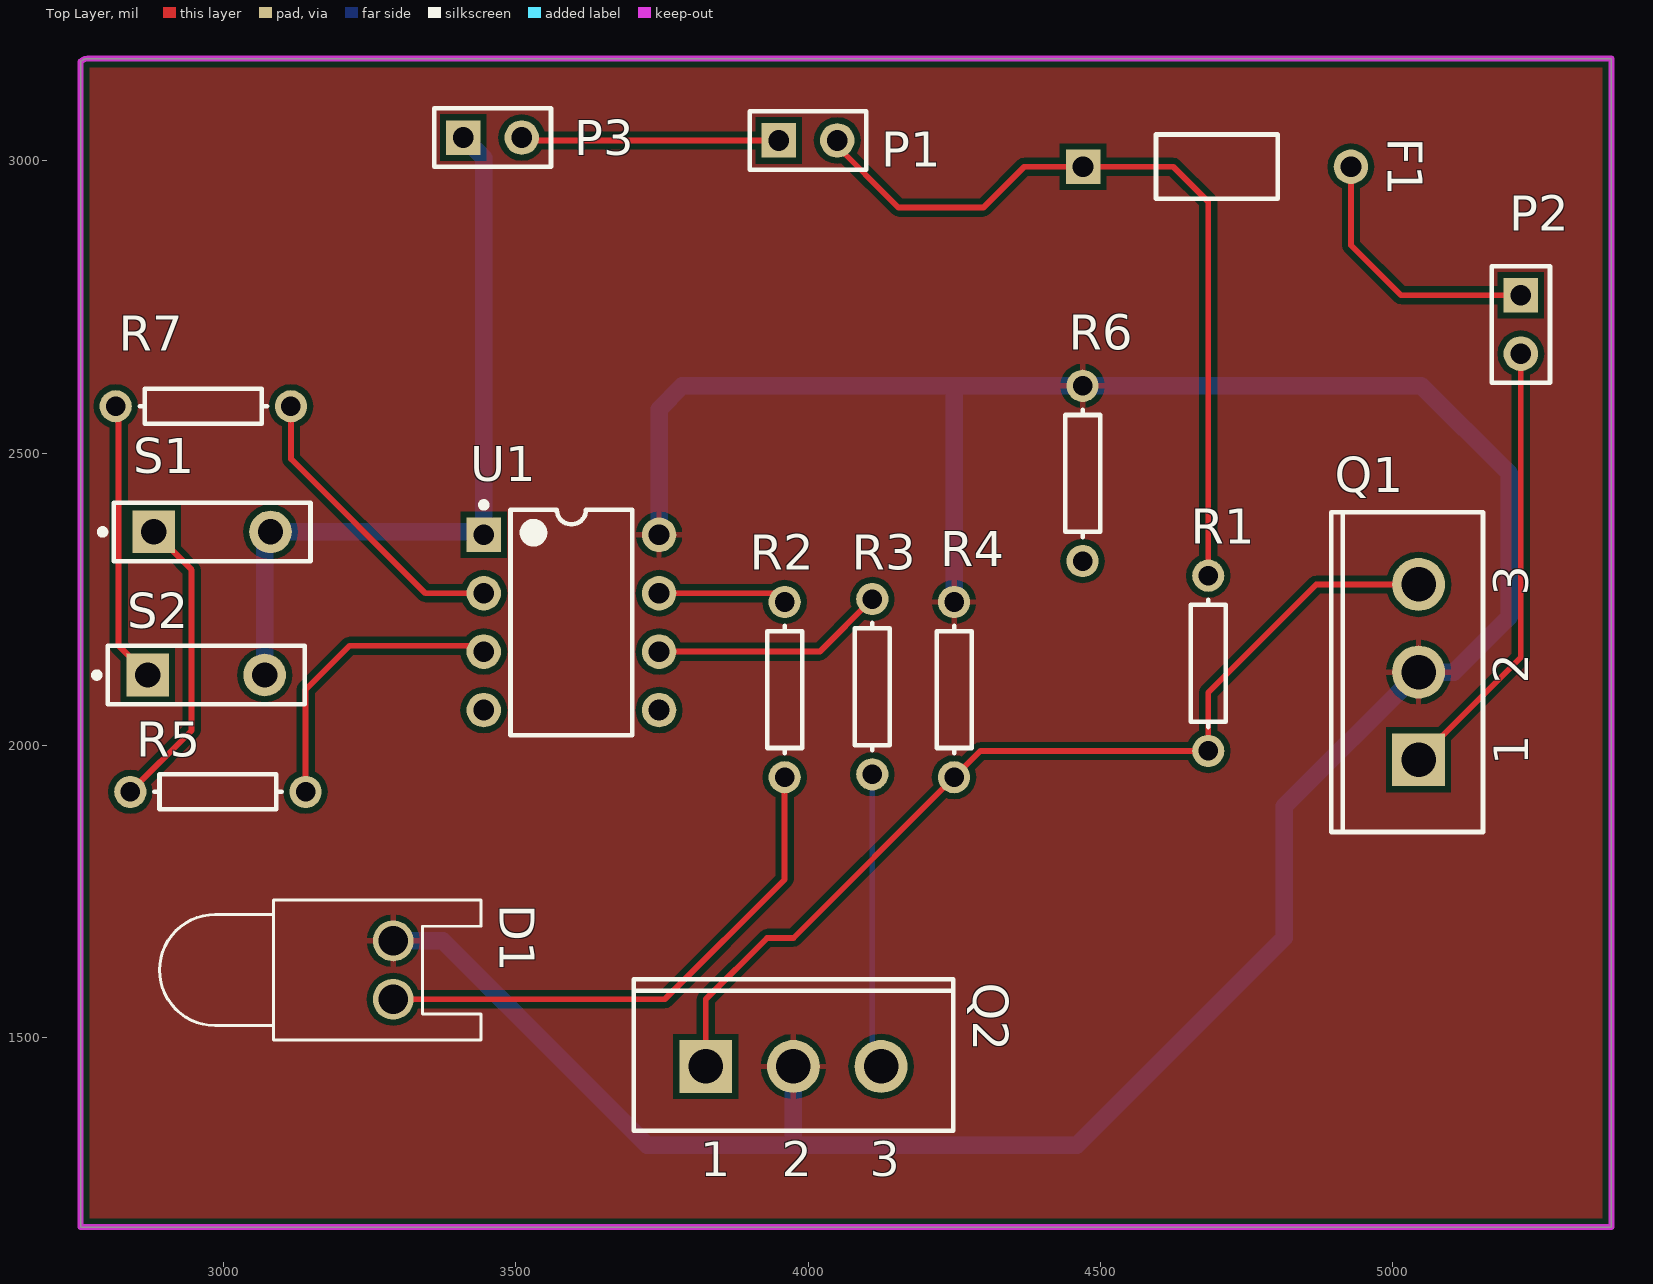
[diagram p0: Top Layer view]
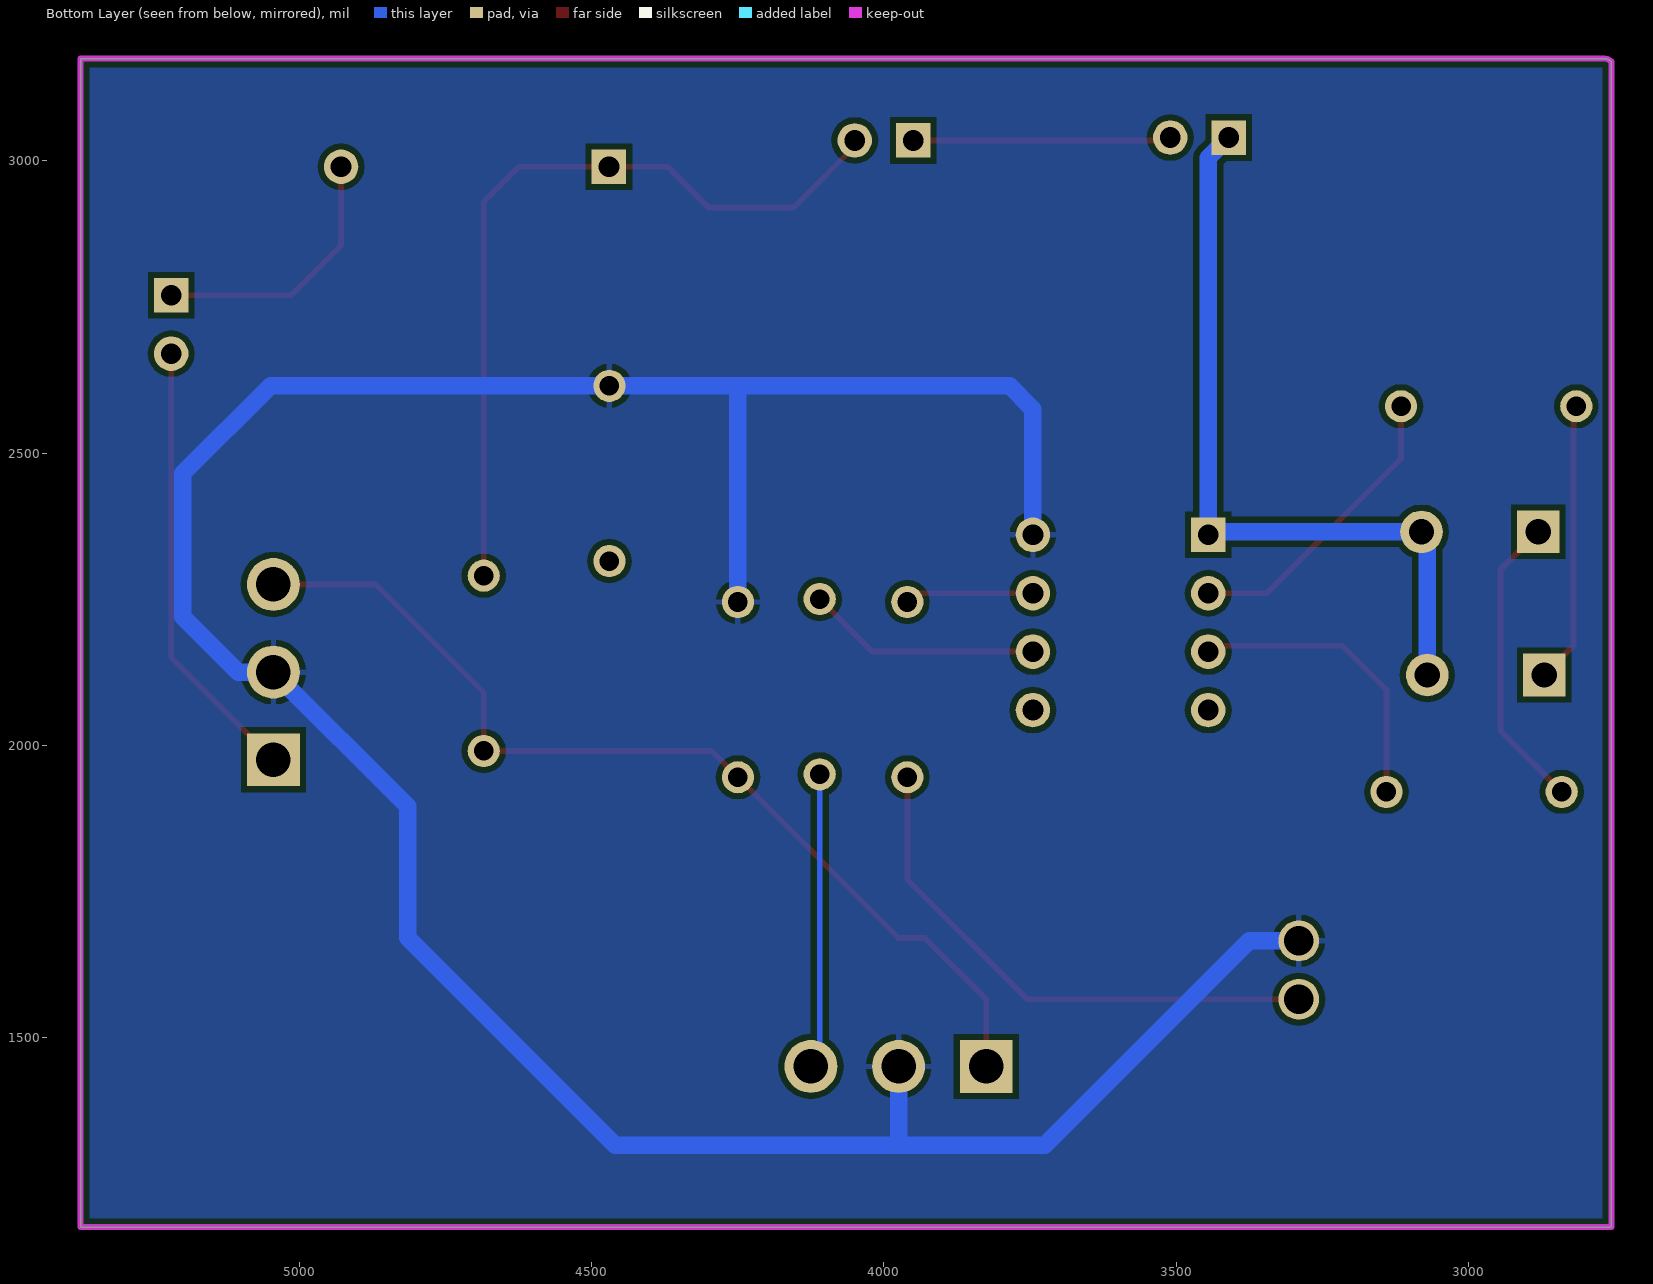
[diagram p1: Bottom Layer view, seen from below]
# Altium PCB MISC80652.PcbDoc
Units mil, origin at the board's own origin, x right, y up, seen from the top; angles counter-clockwise.
Board outline 2620 x 2000 mil, 2 copper layers (Top Layer, Bottom Layer); 17 components, 15 nets, 42 pads, 0 vias.

## Layer stack, top to bottom (the 12.6 mil dielectric is the usual default, probably not edited)
Top Solder: solder mask 0.4, Solder Resist, Dk 3.5
Top Layer: signal copper 1.4
Dielectric 1: dielectric 12.6, FR-4, Dk 4.8
Bottom Layer: signal copper 1.4
Bottom Solder: solder mask 0.4, Solder Resist, Dk 3.5

## Board outline
2755,1175 5375,1175 5375,3175 2767.07,3175 ccw(c2767.07,3157.93) 2755,3170

## Design rules (kind name [scope] priority, off if disabled: settings)
Clearance [All] p1: gap=10
MinimumSolderMaskSliver [All] p1: minsoldermaskwidth=0
PolygonConnect [All] p1: connectstyle=Relief reliefconductorwidth=10 reliefentries=4 polygonreliefangle="90 Angle" airgapwidth=10
RoutingVias [All] p1: holewidth=28 width=50 viastyle="Through Hole" minholewidth=28 minwidth=50 maxholewidth=28 maxwidth=50
SilkToSilkClearance [All] p1: silktosilkclearance=0
SilkToSolderMaskClearance [IsPad] p1: minsilkscreentomaskgap=0 clearancetoexposedcopper=TRUE
SolderMaskExpansion [All] p1: expansion=4
Width [All] p1: maxlimit=30 minlimit=10 preferedwidth=10
27 further rules are at their usual default settings.

## Components (designator, comment, footprint, x,y, rotation, side; value= is the part's Value field where it differs from the comment)
D1 "LED0" LED-0 3290,1615 r270 top
F1 "24V" PIN-W2/E2.8 4700,2990 r0 top
P1 "24VINPUT" HDR1X2 3950,3035 r0 top
P2 "POW OUTPUT" HDR1X2 5220,2770 r270 top
P3 "5VINPUT" HDR1X2 3410,3040 r0 top
Q1 "JANTXV2N7224" TO-254AA 5045,2125 r90 top
Q2 "JANTXV2N7224" TO-254AA 3975,1450 r0 top
R1 "220" AXIAL-0.3 4685,2140 r270 top
R2 "150" AXIAL-0.3 3960,2095 r270 top
R3 "100" AXIAL-0.3 4110,2100 r270 top
R4 "47K" AXIAL-0.3 4250,2095 r90 top
R5 "10K" AXIAL-0.3 2990,1920 r180 top
R6 "10K" AXIAL-0.3 4470,2465 r90 top
R7 "10K" AXIAL-0.3 2965,2580 r180 top
S1 "SW-SPST" SPST-2 2980,2365 r0 top
S2 "SW-SPST" SPST-2 2970,2120 r0 top
U1 "PIC12F508-E/P" PDIP300-P8 3595,2210 r0 top

## Footprints (in the part's own frame and the unit in brackets; to place one, negate y for a bottom-side part, rotate by r counter-clockwise, add the part's x,y. Pads: shape width x height; smd on the part's side, far side on the other; paste and mask are expansions set on the pad)
AXIAL-0.3 [mm] "Axial Device, Thru-Hole; 2 Leads; 0.3 in Pin Spacing"
  round 1.4 hole 0.85: 1(-3.81,0) 2(3.81,0)
  silkscreen extent -2.77,-0.76 2.77,0.76
HDR1X2 [mm] "Connector; Header; 2 Position"
  rect 1.5x1.5 hole 0.9: 1(0,0)
  round 1.5 hole 0.9: 2(2.54,0)
  silkscreen extent -1.27,-1.27 3.81,1.27
LED-0 [mil] "LED; 2 Leads"
  round 70 hole 50: 1(50,0) 2(-50,0)
  silkscreen extent -120,-400 120,150
PDIP300-P8 [mm] "DIP, 8-Leads, Row Spacing 7.62mm, Pitch 2.54mm, Body 9.5x6.6mm"
  rect 1.5x1.5 hole 0.9: 1(-3.81,3.81)
  round 1.5 hole 0.9: 2(-3.81,1.27) 3(-3.81,-1.27) 4(-3.81,-3.81) 5(3.81,-3.81) 6(3.81,-1.27) 7(3.81,1.27) 8(3.81,3.81)
  silkscreen extent -3.93,-4.9 2.65,5.23, body extent -3.55,-4.9 3.55,4.9, height 5.34
PIN-W2/E2.8 [mm] "Thru-Hole; 2 Leads"
  rect 1.5x1.5 hole 0.9: 1(-5.825,0)
  round 1.5 hole 0.9: 2(5.825,0)
  silkscreen extent -2.65,-1.4 2.65,1.4
SPST-2 [mm] "Switch; 2 Leads"
  rect 1.85x1.85 hole 1.1: 1(-2.54,0)
  round 1.85 hole 1.1: 2(2.54,0)
  silkscreen extent -4.89,-1.27 4.28,1.27
TO-254AA [mm] "TO, Thru-Hole, Vertical, Heatsink Mounted; 3 In-Line Leads; Pitch 3.81 mm"
  rect 2.3x2.3 hole 1.5: 1(-3.81,0)
  round 2.3 hole 1.5: 2(0,0) 3(3.81,0)
  silkscreen extent -6.95,-2.8 6.95,3.8

## Part data
D1: "Typical INFRARED GaAs LED"
F1: library part "Fuse 1", "Fuse"
P1 P2 P3: library part "Header 2", "Header, 2-Pin"
Q1 Q2: "HEXFET Power MOSFET"
R1 R2 R3 R4 R5 R6 R7: library part Res1, "Resistor"
S1 S2: "Single-Pole, Single-Throw Switch"
U1: "8-bit Flash Microcontroller, 512 (x12-Bit words) Program Memory, 25 Bytes Data Memory, 8-Pin PDIP, Extended Temperature"

## Nets (pads, with @x,y where several pads share a name; then routed paths per layer and width w, separated by ;. In a path a pad name is that pad's centre, name@x,y a point inside that pad or via, vN(x,y) a via of type N, cw(c..) or ccw(c..) an arc to the next point about the centre after c; other vN are vias at no path point)
5V: P3.1 S1.2 S2.2 U1.1 | length 1310.7
  Bottom Layer w30: S2.2 3070,2355 S1.2 3440,2365 U1.1 3445,3005 P3.1
GND: D1.2 Q1.2 Q2.2 R4.2 R6.2 U1.8 | length 5066.6
  Bottom Layer w30: D1.2 3375,1665 3725,1315 3985,1315 ; U1.8 3745,2575 3785,2615 4255,2615 ; Q2.2 3975,1325 3985,1315 ; R4.2 4250,2610 4255,2615 ; 3985,1315 4460,1315 4815,1670 4815,1895 Q1.2 5105,2125 5200,2220 5200,2465 5050,2615 R6.2 4255,2615
NetD1_1: D1.1 R2.2 | length 929.9
  Top Layer w10: D1.1 3755,1565 3960,1770 R2.2
NetF1_1: F1.1 P1.2 R1.1 | length 1386.5
  Top Layer w10: P1.2@4040,3035 4155,2920 4300,2920 4370,2990 F1.1 4625,2990 4685,2930 R1.1
NetF1_2: F1.2 P2.1 | length 460.5
  Top Layer w10: F1.2 4929.33,2855.67 5015,2770 P2.1
NetP1_1: P1.1 P3.2 | length 442.1
  Top Layer w10: P3.2 3515,3035 P1.1
NetP2_2: P2.2 Q1.1 | length 767.5
  Top Layer w10: Q1.1 5220,2150 P2.2
NetQ1_3: Q1.3 Q2.1 R1.2 R4.1 | length 1687.7
  Top Layer w10: Q2.1 3825,1565 3930,1670 3975,1670 R4.1 4295,1990 R1.2 4685,2090 4870,2275 Q1.3
NetQ2_3: Q2.3 R3.2 | length 506.2
  Bottom Layer w10: R3.2 4110,1465 Q2.3
NetR2_1: R2.1 U1.7 | length 221.2
  Top Layer w10: U1.7 3945,2260 R2.1
NetR3_1: R3.1 U1.6 | length 402.3
  Top Layer w10: U1.6 4020,2160 R3.1
NetR5_1: R5.1 U1.3 | length 515.2
  Top Layer w10: R5.1 3140,2095 3215,2170 3435,2170 U1.3
NetR5_2: R5.2 S1.1 | length 515.4
  Top Layer w10: R5.2 2945,2025 2945,2300 S1.1
NetR7_1: R7.1 U1.2 | length 515.3
  Top Layer w10: R7.1 3115,2490 3345,2260 U1.2
NetR7_2: R7.2 S2.1 | length 482.8
  Top Layer w10: R7.2 2820,2575 2820,2170 S2.1
pads on no net: R6.1 U1.4 U1.5

## Polygon pours and split planes (outlines as drawn)
GND on Bottom Layer "D" (solid, remove dead copper, pour order 0): 2525,3450 2560,3485 6090,3485 6090,1625 5620,1155 5590,1125 2325,1125
GND on Top Layer "D" (solid, remove dead copper, pour order 2): 2425,3425 5450,3425 5615,3590 5560,3535 5560,825 2520,825 2250,1095

## Keep-outs
Keep-Out Layer:
  the board outline again, w10